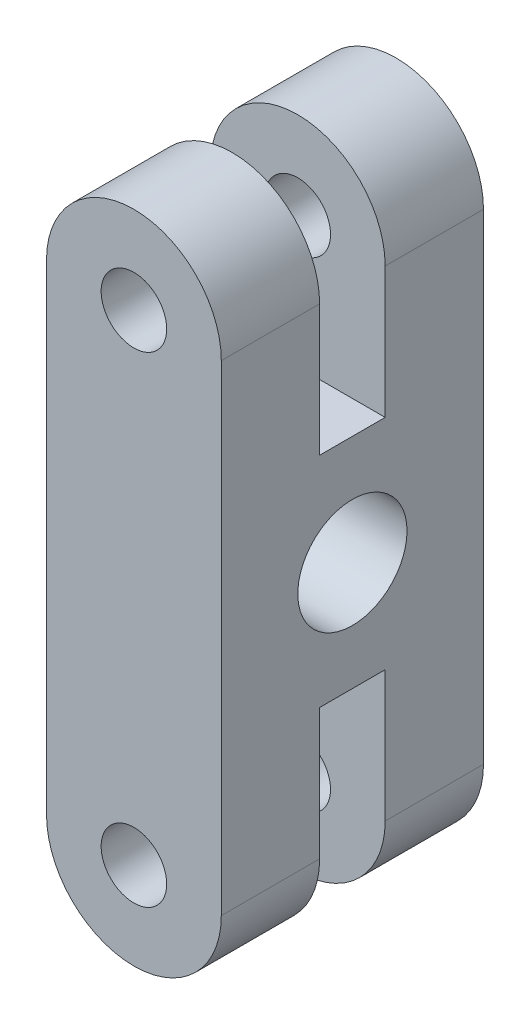
SolidWorks part; units mm, degrees
ref_plane "Front Plane" through (0, 0, 0) normal (0, 0, 1) x (1, 0, 0)
ref_plane "Top Plane" through (0, 0, 0) normal (0, 1, 0) x (1, 0, 0)
ref_plane "Right Plane" through (0, 0, 0) normal (1, 0, 0) x (0, 0, -1)
other "Configuration Table"
sketch "Sketch1" plane through (0, 0, 0) normal (0, 0, 1) x (1, 0, 0)
  line L0 (0, 0) -> (0, 22) construction
  line L1 (-4, 0) -> (-4, 22)
  line L2 (4, 0) -> (4, 22)
  arc A0 (-4, 0) -> (4, 0) centre (0, 0) ccw
  arc A1 (4, 22) -> (-4, 22) centre (0, 22) ccw
  point P3 (0, 11)
  dimension "D1" = 22
  dimension "D2" = 8
extrude "Boss-Extrude1" add sketch "Sketch1" along normal blind 12
sketch "Sketch2" plane through (-4, 0, 0) normal (-1, 0, 0) x (0, 0, 1)
  line L0 (12, 26) -> (0, 26) construction
  line L1 (4.5, 36) -> (7.5, 36)
  line L2 (4.5, 36) -> (4.5, 16)
  line L3 (4.5, 16) -> (7.5, 16)
  line L4 (7.5, 36) -> (7.5, 16)
  line L5 (4.5, 36) -> (7.5, 16) construction
  line L6 (4.5, 16) -> (7.5, 36) construction
  line L7 (0, 11) -> (26.0389, 11) construction
  line L8 (0, 22) -> (0, 0) construction
  line L9 (4.5, -14) -> (7.5, -14)
  line L10 (7.5, -14) -> (7.5, 6)
  line L11 (4.5, -14) -> (4.5, 6)
  line L12 (4.5, 6) -> (7.5, 6)
  point P0 (6, 26)
  dimension "D1" = 3
  dimension "D2" = 10
extrude "Cut-Extrude1" cut sketch "Sketch2" against normal through all
sketch "Sketch3" plane through (0, 0, 12) normal (0, 0, 1) x (1, 0, 0)
  circle A0 centre (0, 22) radius 1.5
  circle A1 centre (0, 0) radius 1.5
  dimension "D1" = 3
extrude "Cut-Extrude2" cut sketch "Sketch3" against normal through all
hole_wizard "M6 Tapped Hole1" positions "3DSketch1" profile "Sketch4" tap size "M6" standard "GB"
sketch3d "3DSketch1"
  line L0 (4, 0, 0) -> (4, 22, 0) construction
  line L1 (4, 6, 7.5) -> (4, 6, 4.5) construction
  point P0 (4, 11, 6)
  dimension "D1" = 6
  dimension "D2" = 5
sketch "Sketch4" plane through (4, 11, 6) normal (0, 1, 0) x (0, 0, -1)
  line L0 (0, 0) -> (0, 7.5022)
  line L1 (0, 7.5022) -> (2.5, 6)
  line L2 (2.5, 6) -> (2.5, 0)
  line L5 (2.5, 0) -> (0, 0)
  line L10 (0, 7.5022) -> (-2.5, 6) construction
  line L11 (0, -6.35) -> (0, 107.95) construction
  dimension "螺纹孔钻头直径" = 5
  dimension "螺纹孔钻头深度" = 6
  dimension "导头角度" = 118
cosmetic thread "Hole thread line 1" parameters "D1"=5, "D2"=6
